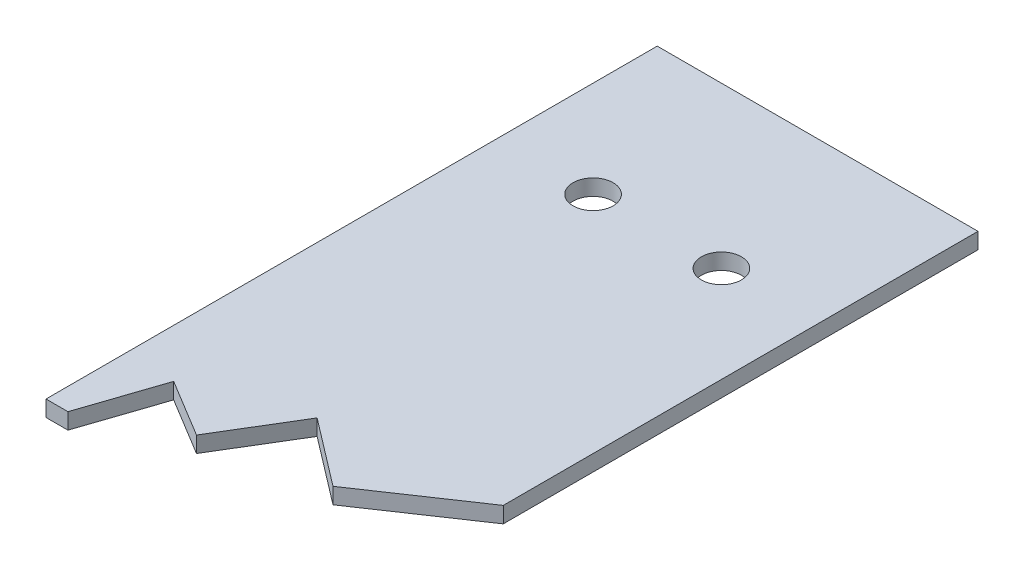
SolidWorks part; units mm, degrees
ref_plane "Front Plane" through (0, 0, 0) normal (0, 0, 1) x (1, 0, 0)
ref_plane "Top Plane" through (0, 0, 0) normal (0, 1, 0) x (1, 0, 0)
ref_plane "Right Plane" through (0, 0, 0) normal (1, 0, 0) x (0, 0, -1)
sketch "Sketch1" plane through (0, 0, 0) normal (0, 1, 0) x (1, 0, 0)
  line L1 (-20, 40) -> (20, 40)
  line L2 (-20, 40) -> (-20, -40)
  line L3 (-20, -40) -> (20, -40)
  line L4 (20, 40) -> (20, -40)
  line L5 (-20, 40) -> (20, -40) construction
  line L6 (-20, -40) -> (20, 40) construction
  point P0 (0, 0)
  dimension "D1" = 40
  dimension "D2" = 80
extrude "Boss-Extrude1" add sketch "Sketch1" along normal blind 2
sketch "Sketch2" plane through (0, 0, 0) normal (0, -1, 0) x (1, 0, 0)
  circle A0 centre (8, -20) radius 2.5
  circle A1 centre (-8, -20) radius 2.5
  dimension "D1" = 5
extrude "Cut-Extrude1" cut sketch "Sketch2" against normal blind 10
sketch "Sketch3" plane through (0, 2, 0) normal (0, 1, 0) x (1, 0, 0)
  line L0 (20, -19.1984) -> (7.3229, -27.7549)
  line L1 (20, -40) -> (20, 40) construction
  line L2 (7.3229, -27.7549) -> (-1.0535, -21.36)
  line L3 (-1.0535, -21.36) -> (-6.7279, -30.7272)
  line L4 (-6.7279, -30.7272) -> (-13.941, -26.3578)
  line L5 (-13.941, -26.3578) -> (-17.266, -36.2214)
  line L6 (-17.266, -36.2214) -> (-20, -36.2214)
  line L7 (-20, 40) -> (-20, -40) construction
  line L8 (-20, -36.2214) -> (-20, -40)
  line L9 (-20, -40) -> (20, -40)
  line L10 (20, -40) -> (20, -19.1984)
extrude "Cut-Extrude2" cut sketch "Sketch3" against normal blind 10
